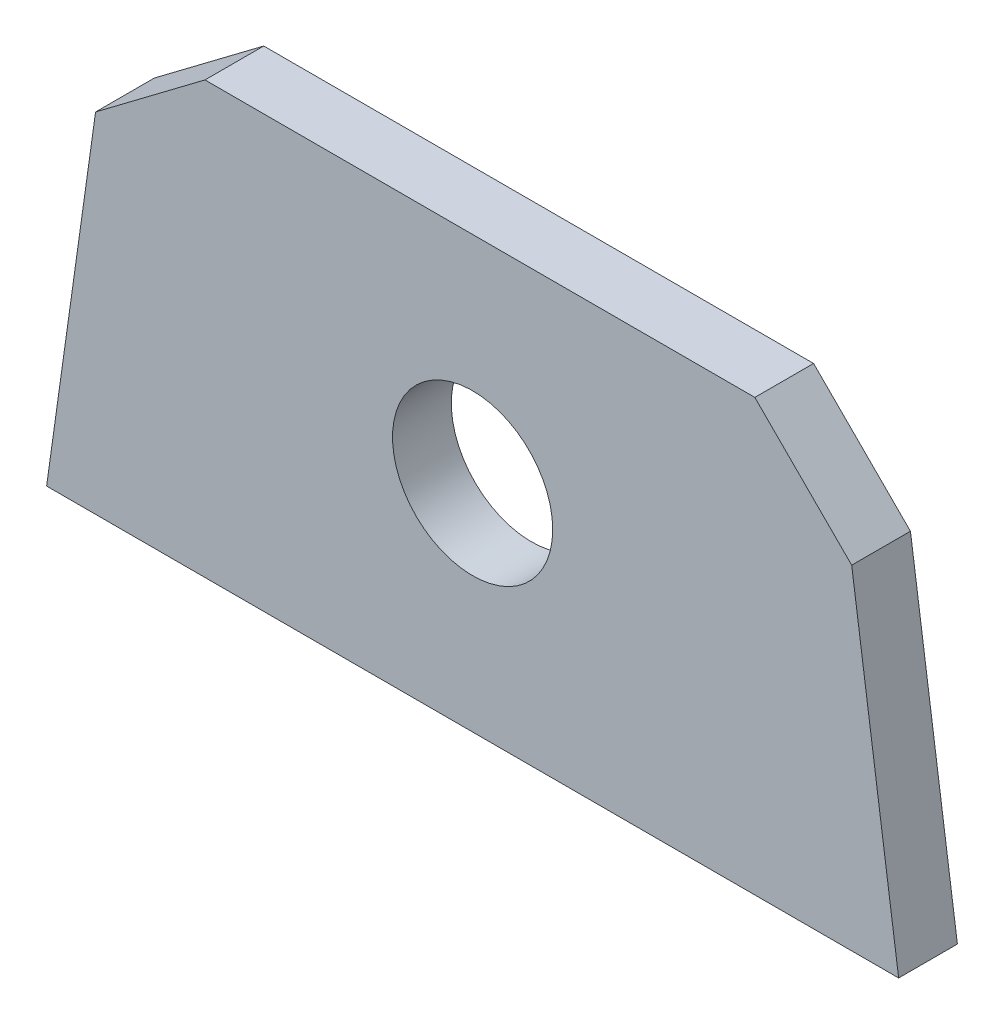
from build123d import *
from OCP.BRepFilletAPI import BRepFilletAPI_MakeChamfer

# Parameters (mm, degrees)
SKETCH_1_W          = 87
SKETCH_1_H          = 44
EXTRUDE_1_DEPTH     = 6
SKETCH_2_R          = 8.179245246
CUT_EXTRUDE_1_DEPTH = 6
CHAMFER_1_SIZE      = 8.5
CHAMFER_1_SIZE2     = 9.987134599


with BuildPart() as part:
    # 草图1 → 凸台-拉伸1 (new body)
    with BuildSketch(Plane.XY):
        Rectangle(SKETCH_1_W, SKETCH_1_H)
    extrude(amount=EXTRUDE_1_DEPTH)

    # 草图2 → 切除-拉伸1 (cut)
    with BuildSketch(Plane.XY.offset(6)):
        Circle(SKETCH_2_R)
        Polygon((-43.5, -22), (-37.316203273, 22), (-43.5, 22), align=None)
        Polygon((43.5, -22), (37.316203273, 22), (43.5, 22), align=None)
    extrude(amount=-CUT_EXTRUDE_1_DEPTH, mode=Mode.SUBTRACT)

    # 倒角1: one chamfer whose edges measure the first distance from different faces: ONE call of the kernel's chamfer builder (chamfer() names one face for all edges)
    chamfer_1_edges_1 = [part.edges().sort_by_distance(p)[0] for p in [
        (37.316203273, 22, 3),
    ]]
    chamfer_1_side_1 = [part.faces().sort_by_distance(p)[0] for p in [
        (0, 22, 3),
    ]]
    chamfer_1_edges_2 = [part.edges().sort_by_distance(p)[0] for p in [
        (-37.316203273, 22, 3),
    ]]
    chamfer_1_side_2 = [part.faces().sort_by_distance(p)[0] for p in [
        (-40.408101637, 0, 3),
    ]]
    chamfer_1 = BRepFilletAPI_MakeChamfer(part.part.solid().wrapped)
    for e in chamfer_1_edges_1:
        chamfer_1.Add(CHAMFER_1_SIZE, CHAMFER_1_SIZE2, e.wrapped, chamfer_1_side_1[0].wrapped)  # the first distance lies on this face
    for e in chamfer_1_edges_2:
        chamfer_1.Add(CHAMFER_1_SIZE, CHAMFER_1_SIZE2, e.wrapped, chamfer_1_side_2[0].wrapped)  # the first distance lies on this face
    add(Compound.cast(chamfer_1.Shape()), mode=Mode.REPLACE)


solid = part.part
